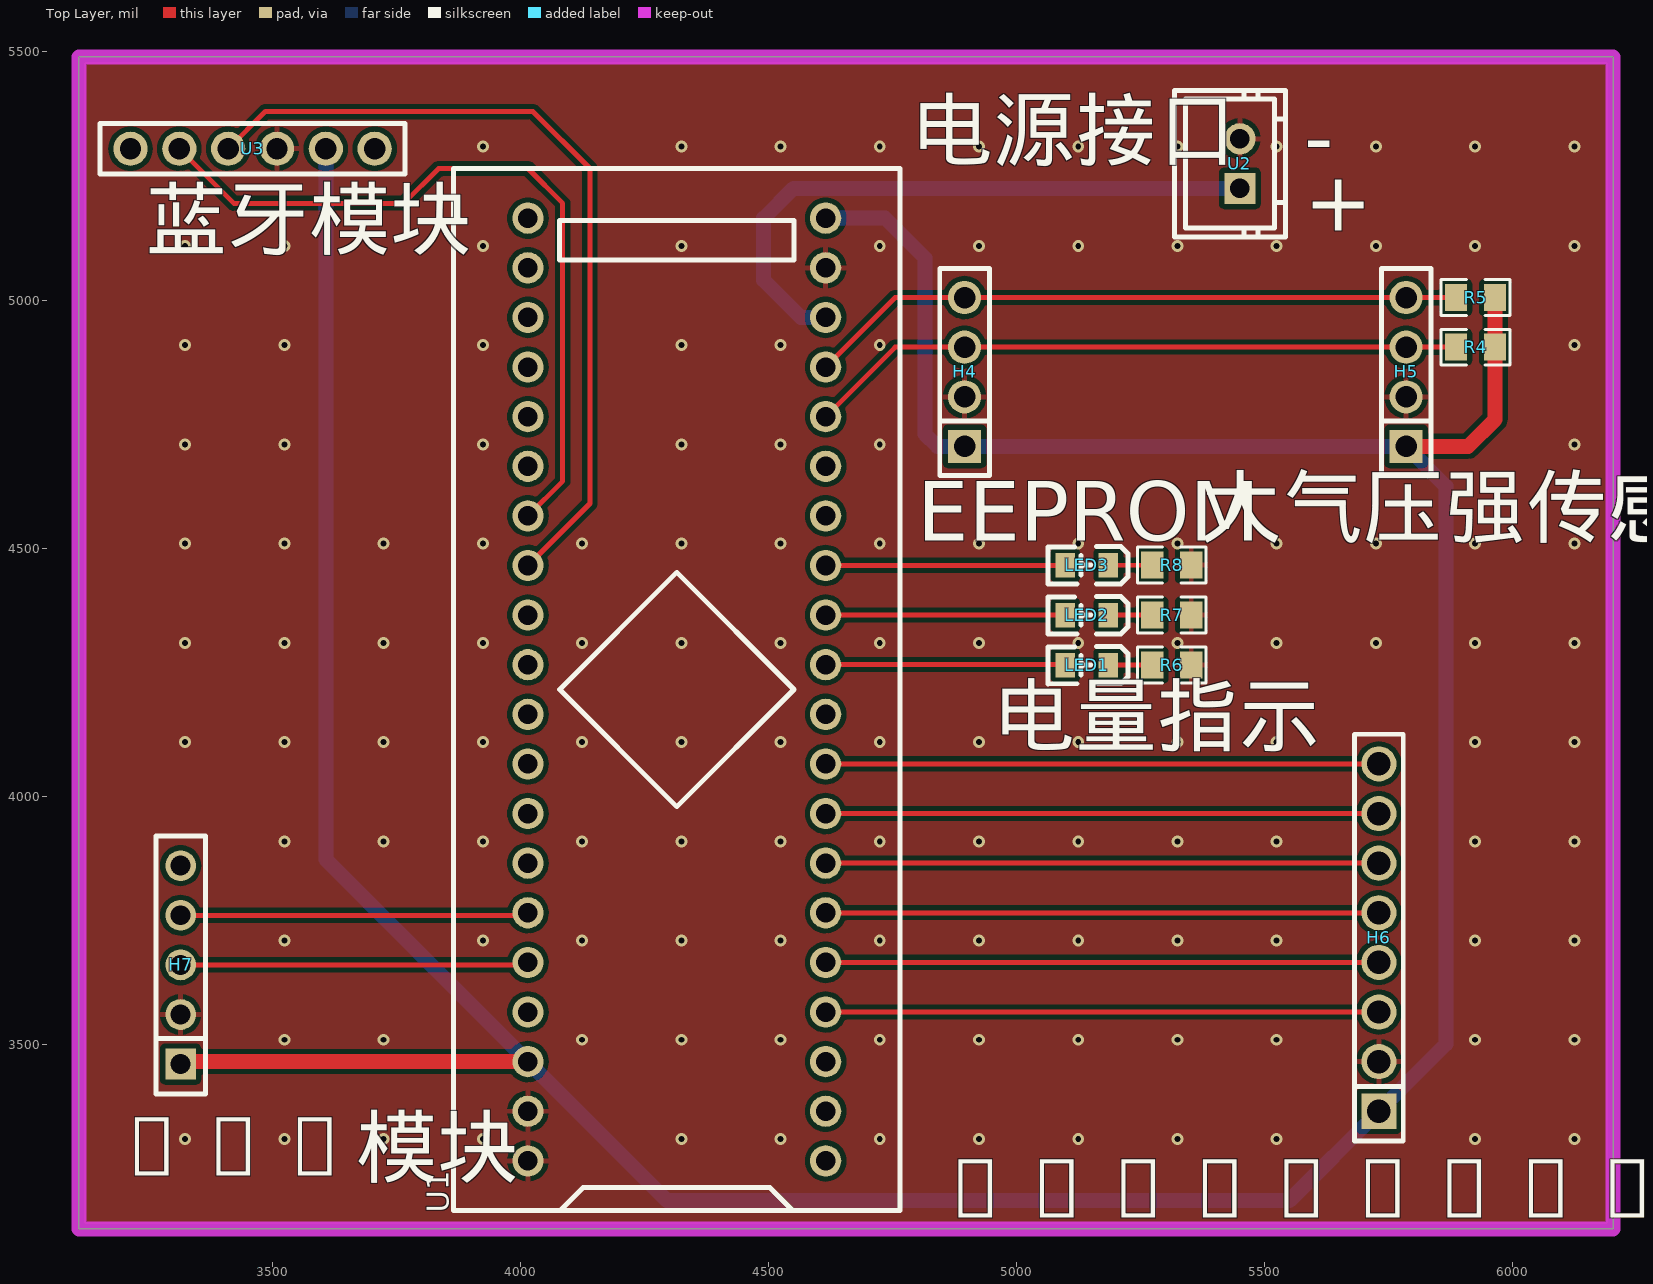
[diagram p0: Top Layer view]
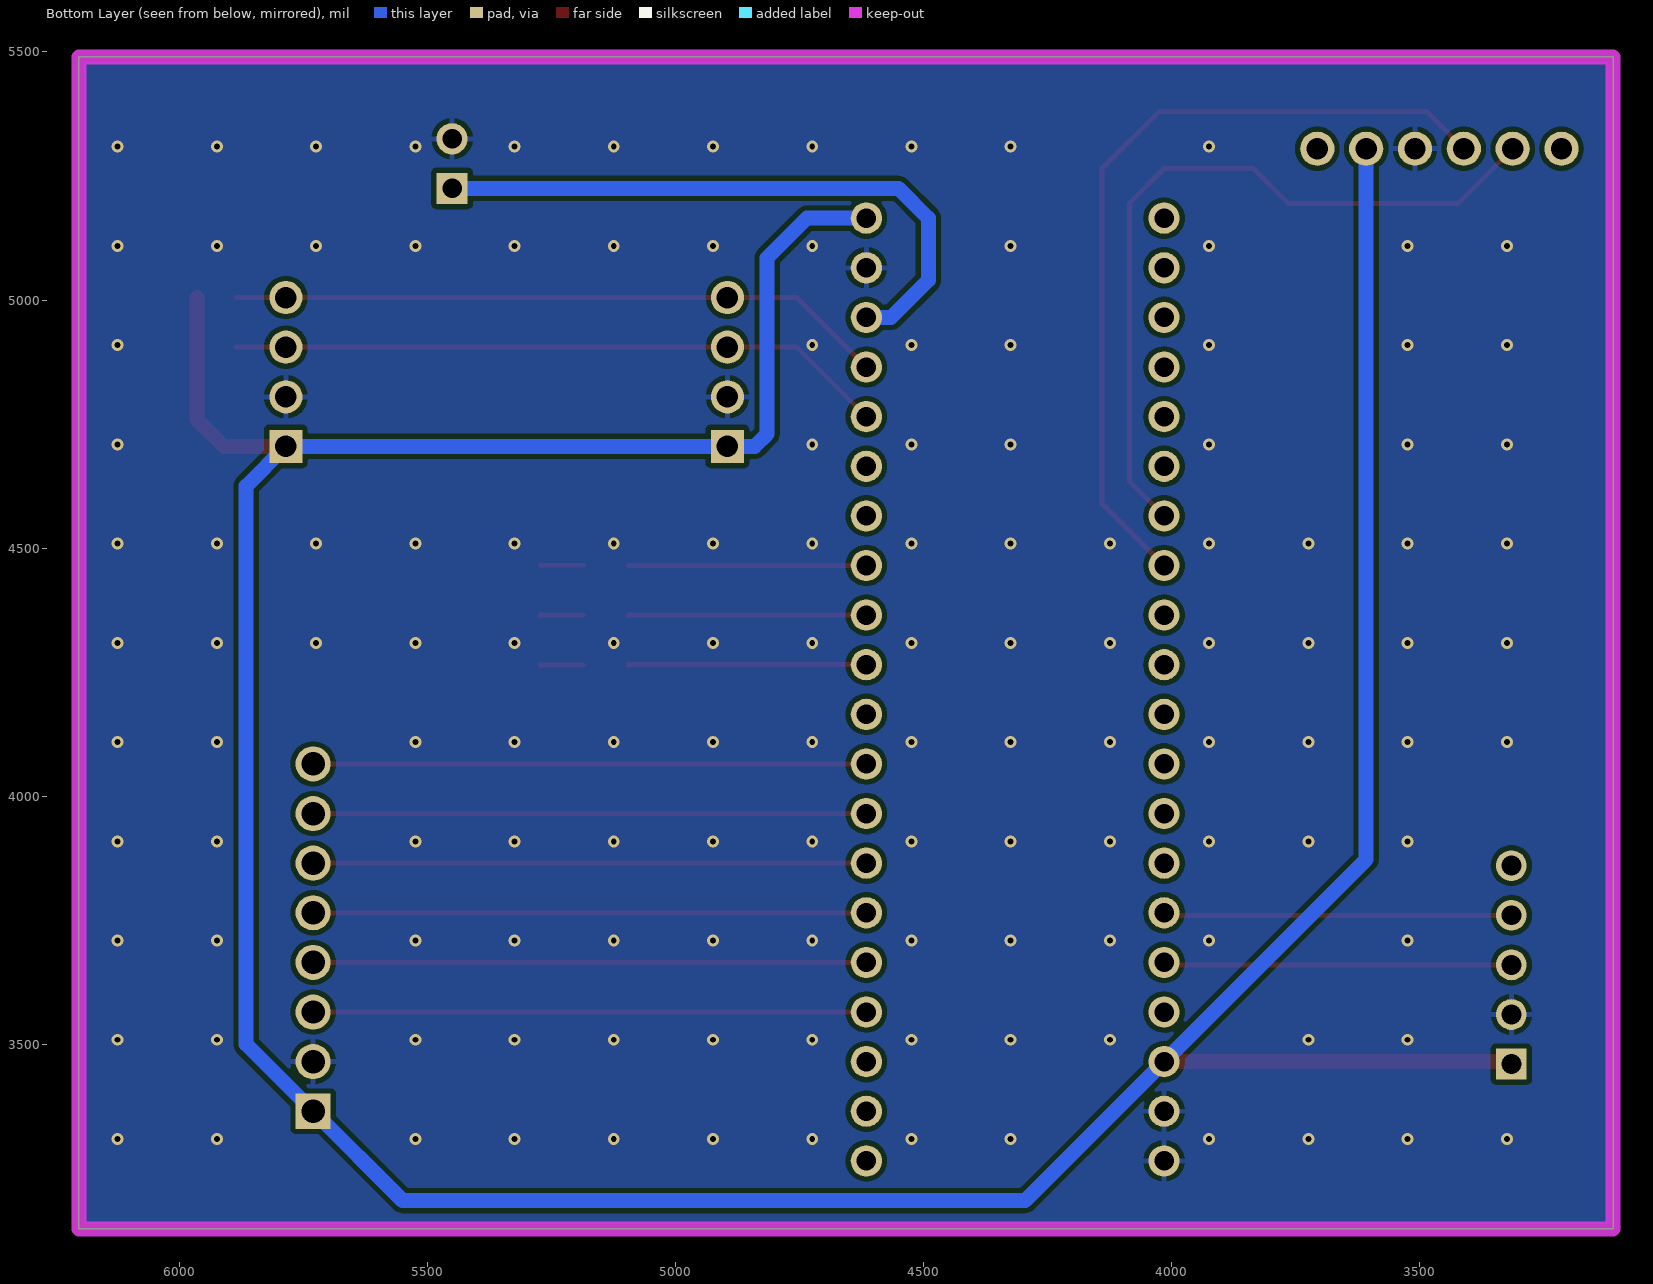
[diagram p1: Bottom Layer view, seen from below]
# Altium PCB MISC51830.pcbdoc
Units mil, origin at the board's own origin, x right, y up, seen from the top; angles counter-clockwise.
Board outline 3092.07 x 2362.2 mil, 2 copper layers (Top Layer, Bottom Layer), stack 62.206 mil thick; 15 components, 24 nets, 85 pads, 131 vias.

## Layer stack, top to bottom
Top Solder Mask Layer: solder mask 0.394, Dk 3.3
Top Layer: signal copper 1.379
Dielectric1: surface 59.449, FR4, Dk 4.5
Bottom Layer: signal copper 1.378
Bottom Solder Mask Layer: solder mask 0.394, Dk 3.3

## Board outline
3110,5490 3110,3127.8 6202.07,3127.8 6202.07,5490

## Design rules (kind name [scope] priority, off if disabled: settings)
BoardOutlineClearance copperThickness2oz_1 [All] p2 off: genericclearance=7.99 ignorepadtopadclearanceinfootprint=FALSE except(0: Arc-SplitContinuation Track-SplitContinuation SMDPad-SplitContinuation THPad-SplitContinuation Via-SplitContinuation Fill-SplitContinuation Region-SplitContinuation Poly-SplitContinuation Text-SplitContinuation Hole-SplitContinuation; 5.98: Arc-CutoutEdge Track-CutoutEdge SMDPad-CutoutEdge THPad-CutoutEdge Via-CutoutEdge Text-CutoutEdge; 6.9: Hole-OutlineEdge Hole-CutoutEdge; 10: Poly-OutlineEdge Poly-CutoutEdge; 11.81: Arc-OutlineEdge Track-OutlineEdge SMDPad-OutlineEdge THPad-OutlineEdge Via-OutlineEdge Fill-OutlineEdge Region-OutlineEdge Text-OutlineEdge Fill-CutoutEdge Region-CutoutEdge)
BoardOutlineClearance Plane_innerPlane_1 [All] p4 off: genericclearance=4.02 ignorepadtopadclearanceinfootprint=FALSE except(0: Arc-SplitContinuation Track-SplitContinuation SMDPad-SplitContinuation THPad-SplitContinuation Via-SplitContinuation Fill-SplitContinuation Region-SplitContinuation Poly-SplitContinuation Text-SplitContinuation Hole-SplitContinuation; 5.98: Arc-CutoutEdge Track-CutoutEdge SMDPad-CutoutEdge THPad-CutoutEdge Via-CutoutEdge Text-CutoutEdge; 6.9: Hole-OutlineEdge Hole-CutoutEdge; 10: Poly-OutlineEdge Poly-CutoutEdge; 11.81: Arc-OutlineEdge Track-OutlineEdge SMDPad-OutlineEdge THPad-OutlineEdge Via-OutlineEdge Fill-OutlineEdge Region-OutlineEdge Text-OutlineEdge Fill-CutoutEdge Region-CutoutEdge)
BoardOutlineClearance Copper_copperRegion_1 [All] p6 off: genericclearance=4.02 ignorepadtopadclearanceinfootprint=FALSE except(0: Arc-SplitContinuation Track-SplitContinuation SMDPad-SplitContinuation THPad-SplitContinuation Via-SplitContinuation Fill-SplitContinuation Region-SplitContinuation Poly-SplitContinuation Text-SplitContinuation Hole-SplitContinuation; 5.98: Arc-CutoutEdge Track-CutoutEdge SMDPad-CutoutEdge THPad-CutoutEdge Via-CutoutEdge Text-CutoutEdge; 6.9: Hole-OutlineEdge Hole-CutoutEdge; 10: Poly-OutlineEdge Poly-CutoutEdge; 11.81: Arc-OutlineEdge Track-OutlineEdge SMDPad-OutlineEdge THPad-OutlineEdge Via-OutlineEdge Fill-OutlineEdge Region-OutlineEdge Text-OutlineEdge Fill-CutoutEdge Region-CutoutEdge)
BoardOutlineClearance copperThickness1oz_1 [All] p8: genericclearance=4.02 ignorepadtopadclearanceinfootprint=FALSE except(0: Arc-SplitContinuation Track-SplitContinuation SMDPad-SplitContinuation THPad-SplitContinuation Via-SplitContinuation Fill-SplitContinuation Region-SplitContinuation Poly-SplitContinuation Text-SplitContinuation Hole-SplitContinuation; 5.98: Arc-CutoutEdge Track-CutoutEdge SMDPad-CutoutEdge THPad-CutoutEdge Via-CutoutEdge Text-CutoutEdge; 6.9: Hole-OutlineEdge Hole-CutoutEdge; 10: Poly-OutlineEdge Poly-CutoutEdge; 11.81: Arc-OutlineEdge Track-OutlineEdge SMDPad-OutlineEdge THPad-OutlineEdge Via-OutlineEdge Fill-OutlineEdge Region-OutlineEdge Text-OutlineEdge Fill-CutoutEdge Region-CutoutEdge)
Clearance copperThickness2oz [All] p1 off: gap=7.99 ignorepadtopadclearanceinfootprint=FALSE except(5.98: SMDPad-Track SMDPad-SMDPad THPad-Track SMDPad-THPad THPad-THPad Track-Via SMDPad-Via THPad-Via Via-Via Fill-SMDPad Region-SMDPad Fill-THPad Region-THPad Fill-Via Region-Via Fill-Fill Fill-Region Region-Region Arc-Track Arc-SMDPad Arc-THPad Arc-Via Fill-Arc Region-Arc Arc-Arc Text-Track SMDPad-Text Text-THPad Text-Via Fill-Text Region-Text Arc-Text Text-Text; 6.9: Hole-Track Hole-SMDPad Hole-THPad Hole-Via Fill-Hole Region-Hole Hole-Arc Hole-Text; 10: Poly-Track Poly-SMDPad Poly-THPad Poly-Via Poly-Fill Poly-Region Poly-Poly Poly-Arc Poly-Text Poly-Hole; 11.81: Fill-Track Region-Track)
Clearance Plane_innerPlane [All] p3 off: gap=4.02 ignorepadtopadclearanceinfootprint=FALSE except(5.98: SMDPad-Track SMDPad-SMDPad THPad-Track SMDPad-THPad THPad-THPad Track-Via SMDPad-Via THPad-Via Via-Via Fill-SMDPad Region-SMDPad Fill-THPad Region-THPad Fill-Via Region-Via Fill-Fill Fill-Region Region-Region Arc-Track Arc-SMDPad Arc-THPad Arc-Via Fill-Arc Region-Arc Arc-Arc Text-Track SMDPad-Text Text-THPad Text-Via Fill-Text Region-Text Arc-Text Text-Text; 6.9: Hole-Track Hole-SMDPad Hole-THPad Hole-Via Fill-Hole Region-Hole Hole-Arc Hole-Text; 10: Poly-Track Poly-SMDPad Poly-THPad Poly-Via Poly-Fill Poly-Region Poly-Poly Poly-Arc Poly-Text Poly-Hole; 11.81: Fill-Track Region-Track)
Clearance Copper_copperRegion [All] p5 off: gap=4.02 ignorepadtopadclearanceinfootprint=FALSE except(5.98: SMDPad-Track SMDPad-SMDPad THPad-Track SMDPad-THPad THPad-THPad Track-Via SMDPad-Via THPad-Via Via-Via Fill-SMDPad Region-SMDPad Fill-THPad Region-THPad Fill-Via Region-Via Fill-Fill Fill-Region Region-Region Arc-Track Arc-SMDPad Arc-THPad Arc-Via Fill-Arc Region-Arc Arc-Arc Text-Track SMDPad-Text Text-THPad Text-Via Fill-Text Region-Text Arc-Text Text-Text; 6.9: Hole-Track Hole-SMDPad Hole-THPad Hole-Via Fill-Hole Region-Hole Hole-Arc Hole-Text; 10: Poly-Track Poly-SMDPad Poly-THPad Poly-Via Poly-Fill Poly-Region Poly-Poly Poly-Arc Poly-Text Poly-Hole; 11.81: Fill-Track Region-Track)
Clearance copperThickness1oz [All] p7: gap=4.02 ignorepadtopadclearanceinfootprint=FALSE except(5.98: SMDPad-Track SMDPad-SMDPad THPad-Track SMDPad-THPad THPad-THPad Track-Via SMDPad-Via THPad-Via Via-Via Fill-SMDPad Region-SMDPad Fill-THPad Region-THPad Fill-Via Region-Via Fill-Fill Fill-Region Region-Region Arc-Track Arc-SMDPad Arc-THPad Arc-Via Fill-Arc Region-Arc Arc-Arc Text-Track SMDPad-Text Text-THPad Text-Via Fill-Text Region-Text Arc-Text Text-Text; 6.9: Hole-Track Hole-SMDPad Hole-THPad Hole-Via Fill-Hole Region-Hole Hole-Arc Hole-Text; 10: Poly-Track Poly-SMDPad Poly-THPad Poly-Via Poly-Fill Poly-Region Poly-Poly Poly-Arc Poly-Text Poly-Hole; 11.81: Fill-Track Region-Track)
DiffPairsRouting differentialPair [All] p1: maxlimit=6 minlimit=6 mostfreqgap=6 toplayer_minwidth=5 toplayer_prefwidth=10 toplayer_maxwidth=100 toplayer_mingap=6 toplayer_prefgap=6 toplayer_maxgap=6 bottomlayer_minwidth=5 bottomlayer_prefwidth=10 bottomlayer_maxwidth=100 bottomlayer_mingap=6 bottomlayer_prefgap=6 bottomlayer_maxgap=6 maxuncoupledlength=10
HoleToHoleClearance otherClearance [All] p1: gap=11.81 allowstackedmicrovias=TRUE
Length netLength [All] p1: minlimit=0 maxlimit=0
PasteMaskExpansion pasteMaskExpansion [All] p1: expansion=0
PlaneConnect innerPlane [All] p1: planeconnectstyle=Relief reliefexpansion=20 reliefentries=4 reliefconductorwidth=10 reliefairgap=10
PolygonConnect copperRegion [All] p1: connectstyle=Relief reliefconductorwidth=10 reliefentries=4 polygonreliefangle="90 Angle" airgapwidth=10 via.connectstyle=Relief via.reliefconductorwidth=10 via.reliefentries=4 via.polygonreliefangle="90 Angle" via.airgapwidth=10
RoutingVias viaSize [All] p1: holewidth=12.01 width=24.02 viastyle="Through Hole" minholewidth=11.81 minwidth=19.68 maxholewidth=248.03 maxwidth=393.7
SolderMaskExpansion solderMaskExpansion [IsVia] p1: expansion=-1000 istentingtop=TRUE
SolderMaskExpansion solderMaskExpansion [All] p2: expansion=2 istentingtop=FALSE
Width copperThickness2oz_2 [All] p1 off: maxlimit=100 minlimit=8 preferedwidth=10
Width copperThickness1oz_2 [All] p2: maxlimit=100 minlimit=5 preferedwidth=10

## Components (designator, comment, footprint, x,y, rotation, side; value= is the part's Value field where it differs from the comment)
H4 "" HDR-TH_4P-P2.54-V-F 4895,4855 r90 top
H5 "" HDR-TH_4P-P2.54-V-F 5785,4855 r90 top
H6 "" HDR-TH_8P-P2.54-V-F-1 5730,3715 r90 top
H7 "" HDR-TH_5P-P2.54-V-F 3315,3660 r90 top
LED1 "" LED_0805 5139.55,4264.26 r180 top
LED2 "" LED_0805 5139.55,4364.98 r180 top
LED3 "" LED_0805 5139.55,4465.69 r180 top
R4 "4.7K" R0805 5925,4905 r180 top
R5 "4.7K" R0805 5925,5005 r180 top
R6 "4.7K" R0805 5312.55,4264.26 r0 top
R7 "4.7K" R0805 5312.55,4364.98 r0 top
R8 "4.7K" R0805 5312.55,4465.69 r0 top
U1 "STM32F103C8T6-Card" CONN-TH_L53.3-W22.9_STM32F103C8T6-CARD 4315,4215 r90 top
U2 "_x001F_XH2.54-2P" CONN-TH_2P-P2.54-V 5450,5275 r90 top
U3 "HC-05_排母*6P" HDR-TH_6P-P2.50-V-F-R1-C6 3460,5305 r0 top

## Footprints (in the part's own frame and the unit in brackets; to place one, negate y for a bottom-side part, rotate by r counter-clockwise, add the part's x,y. Pads: shape width x height; smd on the part's side, far side on the other; paste and mask are expansions set on the pad)
CONN-TH_2P-P2.54-V [mm]
  rect 1.6x1.6 hole 1: 1(-1.27,0)
  round 1.6 hole 1: 2(1.27,0)
  silkscreen extent -3.75,-2.34 3.75,3.36
CONN-TH_L53.3-W22.9_STM32F103C8T6-CARD [mm]
  round 1.6 hole 1: 1(-24.13,-7.62) 2(-21.59,-7.62) 3(-19.05,-7.62) 4(-16.51,-7.62) 5(-13.97,-7.62) 6(-11.43,-7.62) 7(-8.89,-7.62) 8(-6.35,-7.62) 9(-3.81,-7.62) 10(-1.27,-7.62) 11(1.27,-7.62) 12(3.81,-7.62) 13(6.35,-7.62) 14(8.89,-7.62) 15(11.43,-7.62) 16(13.97,-7.62) 17(16.51,-7.62) 18(19.05,-7.62) 19(21.59,-7.62) 20(24.13,-7.62) 21(24.13,7.62) 22(21.59,7.62) 23(19.05,7.62) 24(16.51,7.62) 25(13.97,7.62) 26(11.43,7.62) 27(8.89,7.62) 28(6.35,7.62) 29(3.81,7.62) 30(1.27,7.62) 31(-1.27,7.62) 32(-3.81,7.62) 33(-6.35,7.62) 34(-8.89,7.62) 35(-11.43,7.62) 36(-13.97,7.62) 37(-16.51,7.62) 38(-19.05,7.62) 39(-21.59,7.62) 40(-24.13,7.62)
  silkscreen extent -26.67,-11.43 26.67,11.43
HDR-TH_4P-P2.54-V-F [mm]
  rect 1.7x1.7 hole 1.1: 1(-3.81,0)
  round 1.7 hole 1.1: 2(-1.27,0) 3(1.27,0) 4(3.81,0)
  silkscreen extent -5.29,-1.27 5.29,1.27
HDR-TH_5P-P2.54-V-F [mil]
  rect 62x62 hole 40.16: 1(-200,0)
  round 62 hole 40.16: 2(-100,0) 3(0,0) 4(100,0) 5(200,0)
  silkscreen extent -260,-50 260,50
HDR-TH_6P-P2.50-V-F-R1-C6 [mm]
  round 1.75 hole 1.1 paste+0 mask+0.05: 1(-6.25,0) 2(-3.75,0) 3(-1.25,0) 4(1.25,0) 5(3.75,0) 6(6.25,0)
  silkscreen extent -7.8,-1.3 7.8,1.3
HDR-TH_8P-P2.54-V-F-1 [mm]
  rect 1.8x1.8 hole 1.2: 1(-8.89,0)
  round 1.8 hole 1.2: 2(-6.35,0) 3(-3.81,0) 4(-1.27,0) 5(1.27,0) 6(3.81,0) 7(6.35,0) 8(8.89,0)
  silkscreen extent -10.41,-1.25 10.41,1.25
LED_0805 [mm]
  rect 1x1.25 smd paste+0 mask+0.051: 1(-1.15,0.005) 2(1.05,0.005)
  silkscreen extent -2.15,-0.94 1.93,0.97
R0805 [mm]
  rect 1.133x1.377 smd paste-100 mask+0.051: 1(-1,0) 2(1,0)
  silkscreen extent -1.76,-0.92 1.76,0.92

## Via types
v1: diameter 24.02, hole 12, Top Layer to Bottom Layer, 131 vias

## Nets (pads, with @x,y where several pads share a name; then routed paths per layer and width w, separated by ;. In a path a pad name is that pad's centre, name@x,y a point inside that pad or via, vN(x,y) a via of type N, cw(c..) or ccw(c..) an arc to the next point about the centre after c; other vN are vias at no path point)
$1N824: LED1.1 R6.1 | length 88.4
  Top Layer w10: LED1.1 5272.98,4264.06 R6.1
$1N874: LED2.1 R7.1 | length 88.4
  Top Layer w10: LED2.1 5272.98,4364.77 R7.1
$1N900: LED3.1 R8.1 | length 88.4
  Top Layer w10: LED3.1 5272.98,4465.49 R8.1
+5V: U1.18 U2.1 | length 1265.9
  Bottom Layer w30: U1.18 4565,4965 4490,5040 4490,5165 4550,5225 U2.1
CS: H6.6 U1.7 | length 1115
  Top Layer w10: U1.7 H6.6
EN: U1.29
GND: H4.2 H5.2 H6.2 H7.2 R6.2 R7.2 R8.2 U1.19 U1.39 U1.40 U2.2 U3.4
  other v1: 3324.1,3309.1 3524.1,3309.1 3724.1,3309.1 3924.1,3309.1 4324.1,3309.1 4524.1,3309.1 4724.1,3309.1 4924.1,3309.1 5124.1,3309.1 5324.1,3309.1 5524.1,3309.1 5924.1,3309.1 6124.1,3309.1 3524.1,3509.1 3724.1,3509.1 4124.1,3509.1 4324.1,3509.1 4524.1,3509.1 4724.1,3509.1 4924.1,3509.1 5124.1,3509.1 5324.1,3509.1 5524.1,3509.1 5924.1,3509.1 6124.1,3509.1 3524.1,3709.1 3924.1,3709.1 4124.1,3709.1 4324.1,3709.1 4524.1,3709.1 4724.1,3709.1 4924.1,3709.1 5124.1,3709.1 5324.1,3709.1 5524.1,3709.1 5924.1,3709.1 6124.1,3709.1 3524.1,3909.1 3724.1,3909.1 3924.1,3909.1 4124.1,3909.1 4324.1,3909.1 4524.1,3909.1 4724.1,3909.1 4924.1,3909.1 5124.1,3909.1 5324.1,3909.1 5524.1,3909.1 5924.1,3909.1 6124.1,3909.1 3324.1,4109.1 3524.1,4109.1 3724.1,4109.1 3924.1,4109.1 4124.1,4109.1 4324.1,4109.1 4524.1,4109.1 4724.1,4109.1 4924.1,4109.1 5124.1,4109.1 5324.1,4109.1 5524.1,4109.1 5924.1,4109.1 6124.1,4109.1 3324.1,4309.1 3524.1,4309.1 3724.1,4309.1 3924.1,4309.1 4124.1,4309.1 4324.1,4309.1 4524.1,4309.1 4724.1,4309.1 4924.1,4309.1 5124.1,4309.1 5324.1,4309.1 5524.1,4309.1 5724.1,4309.1 5924.1,4309.1 6124.1,4309.1 3324.1,4509.1 3524.1,4509.1 3724.1,4509.1 3924.1,4509.1 4124.1,4509.1 4324.1,4509.1 4524.1,4509.1 4724.1,4509.1 4924.1,4509.1 5124.1,4509.1 5324.1,4509.1 5524.1,4509.1 5724.1,4509.1 5924.1,4509.1 6124.1,4509.1 3324.1,4709.1 3524.1,4709.1 3924.1,4709.1 4324.1,4709.1 4524.1,4709.1 4724.1,4709.1 6124.1,4709.1 3324.1,4909.1 3524.1,4909.1 3924.1,4909.1 4324.1,4909.1 4524.1,4909.1 4724.1,4909.1 6124.1,4909.1 3324.1,5109.1 3524.1,5109.1 3924.1,5109.1 4324.1,5109.1 4724.1,5109.1 4924.1,5109.1 5124.1,5109.1 5324.1,5109.1 5524.1,5109.1 5724.1,5109.1 5924.1,5109.1 6124.1,5109.1 3924.1,5309.1 4324.1,5309.1 4524.1,5309.1 4724.1,5309.1 4924.1,5309.1 5124.1,5309.1 5324.1,5309.1 5524.1,5309.1 5724.1,5309.1 5924.1,5309.1 6124.1,5309.1
INT1: H6.7 U1.8 | length 1115
  Top Layer w10: U1.8 H6.7
INT2: H6.8 U1.9 | length 1115
  Top Layer w10: U1.9 H6.8
MISO: H6.3 U1.4 | length 1115
  Top Layer w10: U1.4 H6.3
MOSI: H6.4 U1.5 | length 1115
  Top Layer w10: U1.5 H6.4
PB3: LED1.2 U1.11 | length 481
  Top Layer w10: U1.11 5094.35,4265 LED1.2@5095.5,4263.85
PB4: LED2.2 U1.12 | length 480.8
  Top Layer w10: U1.12 5094.75,4365 LED2.2@5095.5,4364.25
PB5: LED3.2 U1.13 | length 480.6
  Top Layer w10: U1.13 5095.15,4465 LED3.2@5095.5,4464.66
PPS: U1.34
RX: H7.4 U1.35 | length 702.1
  Top Layer w10: H7.4 4010,3760 U1.35
RXD: U1.27 U3.2 | length 1535.2
  Top Layer w10: U3.2 3422.36,5195 3765,5195 3835,5265 4015,5265 4085,5195 4085,4635 U1.27
SCL: H4.3 H5.3 R4.2 U1.16 | length 1328.6
  Top Layer w10: U1.16 4755,4905 H4.3 H5.3 R4.2
SCLK: H6.5 U1.6 | length 1115
  Top Layer w10: U1.6 H6.5
SDA: H4.4 H5.4 R5.2 U1.17 | length 1328.6
  Top Layer w10: U1.17 4755,5005 H4.4 H5.4 R5.2
STATE: U1.26
TX: H7.3 U1.36 | length 702.1
  Top Layer w10: H7.3 4010,3660 U1.36
TXD: U1.28 U3.3 | length 1659.7
  Top Layer w10: U3.3 3485.79,5380 4025,5380 4140,5265 4140,4590 U1.28
VCC: H4.1 H5.1 H6.1 H7.1 R4.1 R5.1 U1.20 U1.38 U3.5 | length 8061.4
  Top Layer w30: H7.1 3320,3465 U1.38 ; H5.1 5910,4705 5964.37,4759.37 R4.1 R5.1
  Bottom Layer w30: U3.5 3607.64,3872.36 U1.38 4295,3185 5550,3185 H6.1 5865,3500 5865,4625 H5.1 H4.1 4840,4705 4815,4730 4815,5085 4735,5165 U1.20
pads on no net: H7.5 U1.1 U1.2 U1.3 U1.10 U1.14 U1.15 U1.21 U1.22 U1.23 U1.24 U1.25 U1.30 U1.31 U1.32 U1.33 U1.37 U3.1 U3.6

## Polygon pours and split planes (outlines as drawn)
GND on Top Layer (solid, remove dead copper, pour order 0): 3010,5600 3010,3020 6375,3020 6375,5600
GND on Bottom Layer (solid, remove dead copper, pour order 2): 3000,5625 3000,3000 6375,3000 6375,5625

## Keep-outs
Board Outline Layer:
  the board outline again, w30

## Silkscreen, mask and mechanical layers (free items; w line width, h text height)
Top Silkscreen Layer:
  text "电源接口" at 4790,5285 h120
  text "-" at 5580,5270 h120
  text "+" at 5580,5140 h120
  text "蓝牙模块" at 3245,5105 h120
  text "大气压强传感器" at 5370,4525 h120
  text "EEPROM" at 4800,4515 h120
  text "电量指示" at 4955,4105 h120
  text "GPS模块" at 3175,3235 h120
  text "BMI270+BMM150六轴加速度" at 4835,3150 h120